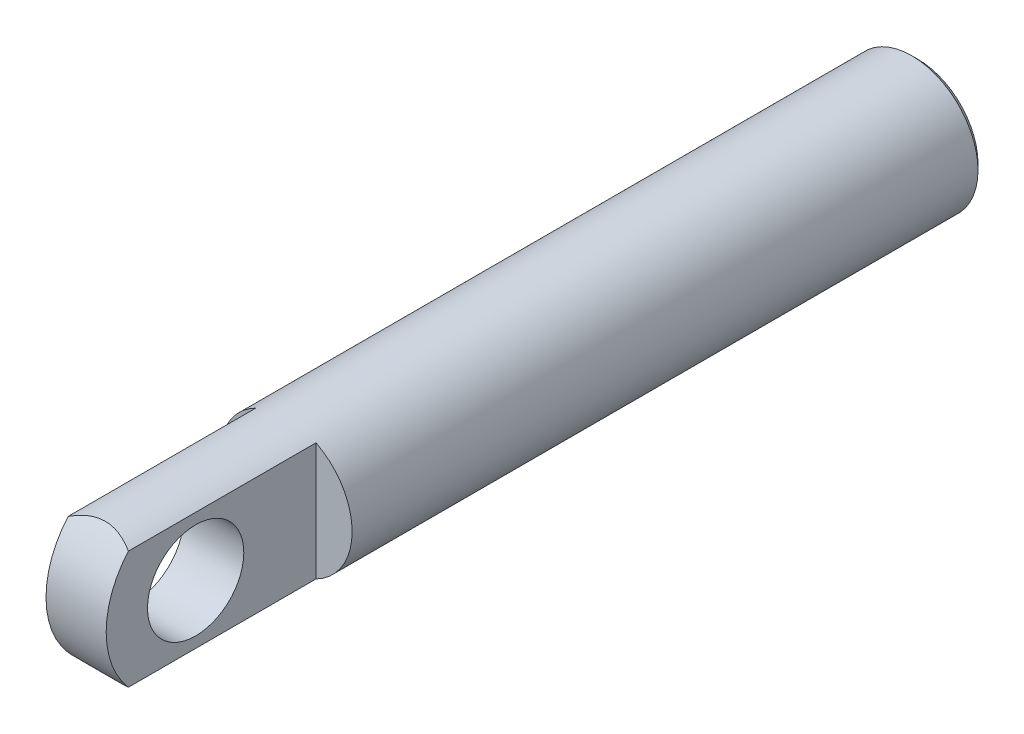
SolidWorks part; units mm, degrees
ref_plane "Front Plane" through (0, 0, 0) normal (0, 0, 1) x (1, 0, 0)
ref_plane "Top Plane" through (0, 0, 0) normal (0, 1, 0) x (1, 0, 0)
ref_plane "Right Plane" through (0, 0, 0) normal (1, 0, 0) x (0, 0, -1)
other "Configuration Table"
sketch "Sketch1" plane through (0, 0, 0) normal (0, 0, 1) x (1, 0, 0)
  circle A0 centre (0, 0) radius 11
  dimension "D1" = 22
extrude "Boss-Extrude1" add sketch "Sketch1" along normal blind 140
sketch "Sketch2" plane through (0, 0, 140) normal (0, 0, 1) x (1, 0, 0)
  line L1 (5, 14.3488) -> (21.8689, 14.3488)
  line L2 (5, 14.3488) -> (5, -18.206)
  line L3 (5, -18.206) -> (21.8689, -18.206)
  line L4 (21.8689, 14.3488) -> (21.8689, -18.206)
  line L5 (-18.3015, 14.6874) -> (-5, 14.6874)
  line L6 (-18.3015, 14.6874) -> (-18.3015, -17.3832)
  line L7 (-18.3015, -17.3832) -> (-5, -17.3832)
  line L8 (-5, 14.6874) -> (-5, -17.3832)
  dimension "D1" = 10
  dimension "D2" = 5
extrude "Cut-Extrude1" cut sketch "Sketch2" against normal blind 35 and the other way through all
hole_wizard "M12x1.5 Tapped Hole1" positions "3DSketch2" profile "Sketch4" tap size "M12x1.5" standard "GB"
sketch3d "3DSketch2"
  point P0 (-0.0003, -0.0004, 0)
sketch "Sketch4" plane through (-0.0003, -0.0004, 0) normal (1, 0, 0) x (0, 1, 0)
  line L0 (0, 0) -> (0, 102.6545)
  line L1 (0, 102.6545) -> (5.25, 99.5)
  line L2 (5.25, 99.5) -> (5.25, 0)
  line L5 (5.25, 0) -> (0, 0)
  line L10 (0, 102.6545) -> (-5.25, 99.5) construction
  line L11 (0, -6.35) -> (0, 107.95) construction
  dimension "螺纹孔钻头直径" = 10.5
  dimension "螺纹孔钻头深度" = 99.5
  dimension "导头角度" = 118
cosmetic thread "Hole thread line 1" parameters "D1"=95, "D2"=12
chamfer "Chamfer1" distance 1 angle 45 1 edges at (11, 0, 0)
sketch "Sketch5" plane through (-5, 0, 0) normal (-1, 0, 0) x (0, 0, 1)
  line L1 (125, 14.8665) -> (182.888, 36.7435)
  line L2 (182.888, 36.7435) -> (236.6735, -7.3492)
  line L3 (236.6735, -7.3492) -> (192.7709, -51.0617)
  line L4 (192.7709, -51.0617) -> (125, -14.8665)
  line L5 (140, 9.798) -> (140, -9.798) construction
  circle A0 centre (125, 0) radius 8
  arc A1 (125, -14.8665) -> (125, 14.8665) centre (125, 0) ccw
  dimension "D1" = 15
  dimension "D2" = 16
extrude "Cut-Extrude2" cut sketch "Sketch5" against normal through all
